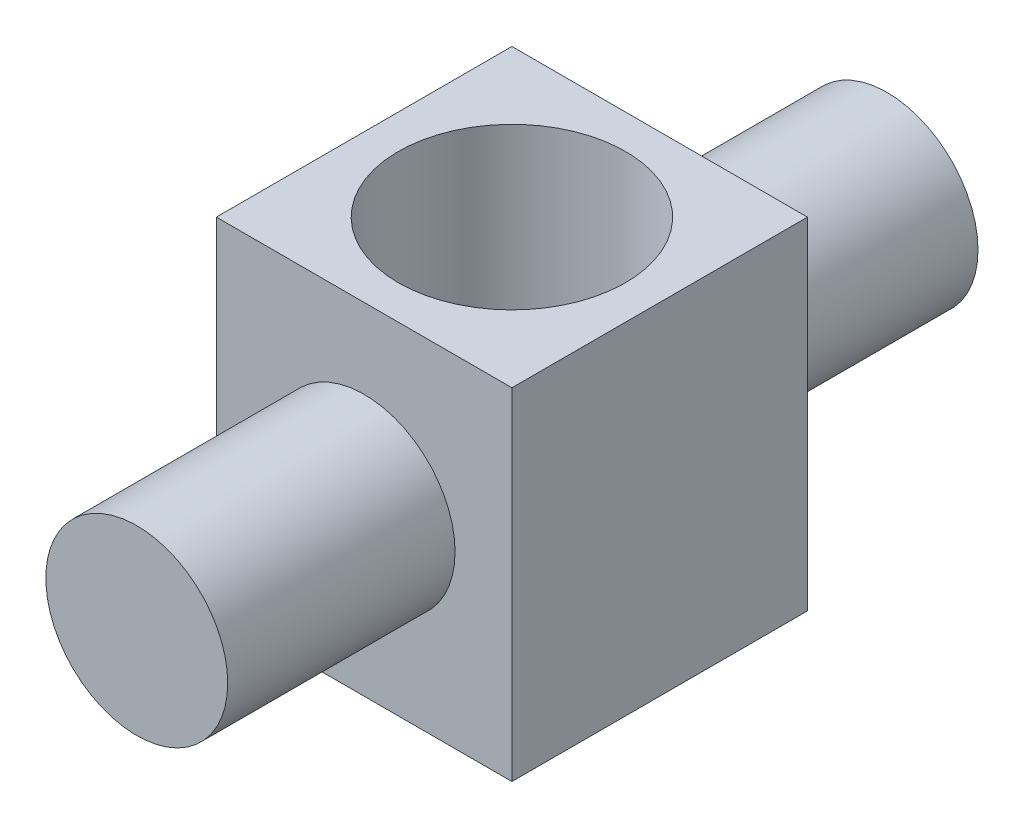
SolidWorks part; units mm, degrees
material "AISI 1045 Steel, cold drawn"
ref_plane "Front Plane" through (0, 0, 0) normal (0, 0, 1) x (1, 0, 0)
ref_plane "Top Plane" through (0, 0, 0) normal (0, 1, 0) x (1, 0, 0)
ref_plane "Right Plane" through (0, 0, 0) normal (1, 0, 0) x (0, 0, -1)
sketch "Sketch1" plane through (0, 0, 0) normal (0, 1, 0) x (1, 0, 0)
  line L1 (-6.5, -6.5) -> (6.5, -6.5)
  line L2 (-6.5, -6.5) -> (-6.5, 6.5)
  line L3 (-6.5, 6.5) -> (6.5, 6.5)
  line L4 (6.5, -6.5) -> (6.5, 6.5)
  line L5 (-6.5, -6.5) -> (6.5, 6.5) construction
  line L6 (-6.5, 6.5) -> (6.5, -6.5) construction
  circle A0 centre (0, 0) radius 5
  point P0 (0, 0)
  dimension "D3" = 10
  dimension "D1" = 13
  dimension "D2" = 13
extrude "Boss-Extrude1" add sketch "Sketch1" along normal mid plane 15
sketch "Sketch2" plane through (0, 0, 6.5) normal (0, 0, 1) x (1, 0, 0)
  circle A0 centre (0, 0) radius 4
  dimension "D1" = 8
extrude "Boss-Extrude2" add sketch "Sketch2" along normal blind 10
mirror "Mirror1" about plane through (0, 0, 0) normal (0, 0, 1) of "Boss-Extrude2"
